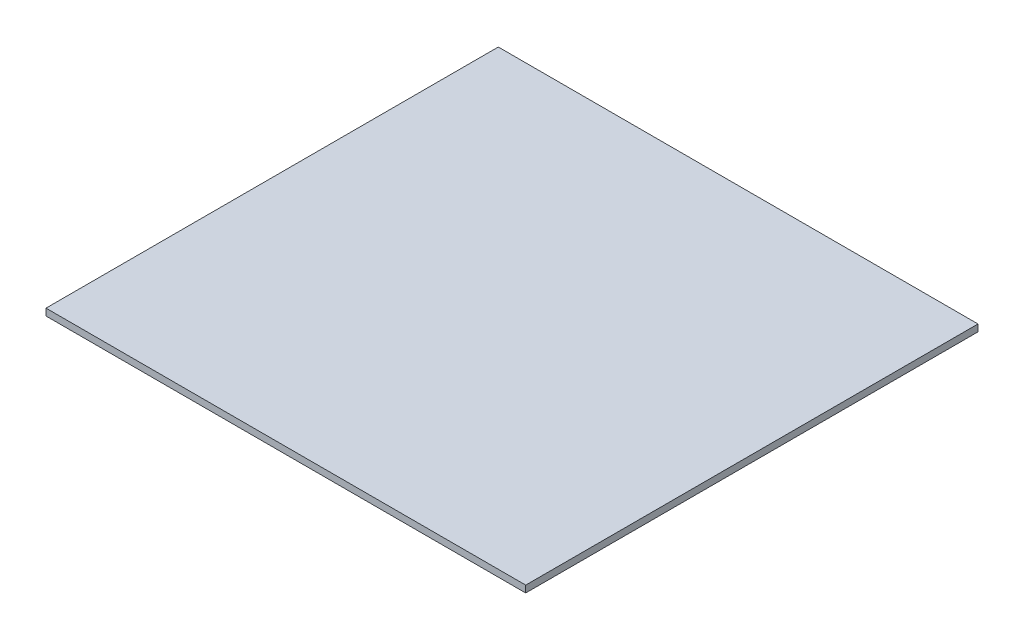
SolidWorks part; units mm, degrees
ref_plane "Front" through (0, 0, 0) normal (0, 0, 1) x (1, 0, 0)
ref_plane "Top" through (0, 0, 0) normal (0, 1, 0) x (1, 0, 0)
ref_plane "Right" through (0, 0, 0) normal (1, 0, 0) x (0, 0, -1)
sketch "Sketch1" plane through (0, 0, 0) normal (0, 1, 0) x (1, 0, 0)
  line L1 (-350, -330) -> (350, -330)
  line L2 (-350, -330) -> (-350, 330)
  line L4 (350, -330) -> (350, 330)
  line L5 (-350, -330) -> (350, 330) construction
  line L6 (-350, 330) -> (350, -330) construction
  line L9 (-350, 330) -> (350, 330)
  point P0 (0, 0)
  point P6 (-350, 370)
  point P7 (350, 370)
  point P8 (310, -330)
  point P9 (310, 370)
  point P10 (-310, -330)
  point P11 (-310, 370)
  dimension "D1" = 700
  dimension "D2" = 660
extrude "Boss-Extrude1" add sketch "Sketch1" along normal blind 10
